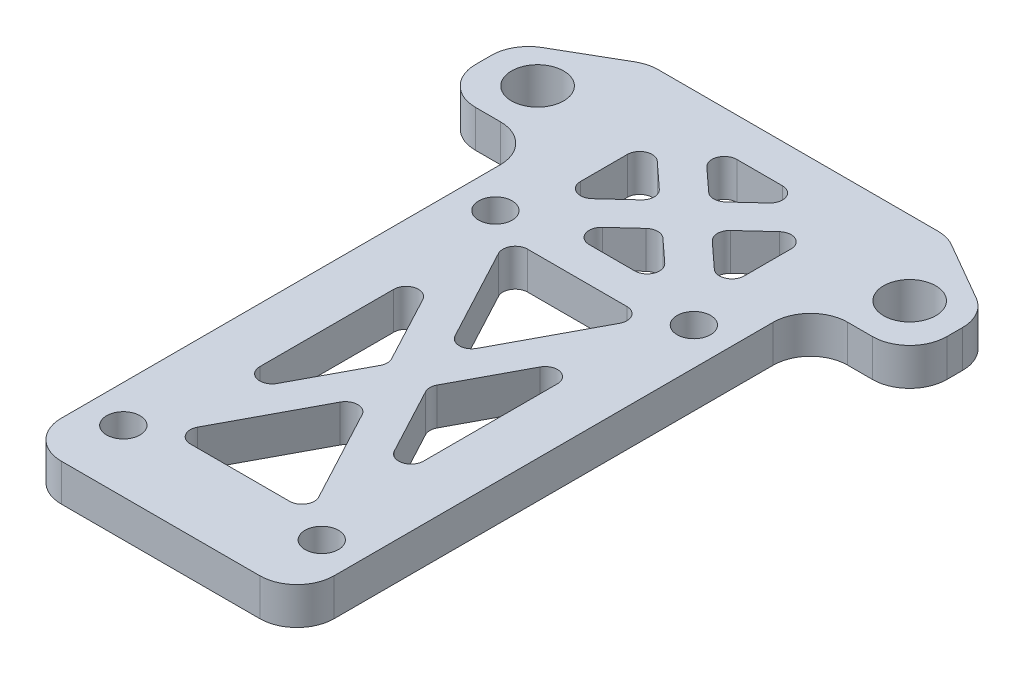
SolidWorks part; units mm, degrees
material "Thornel Mat VMA"
ref_plane "前视基准面" through (0, 0, 0) normal (0, 0, 1) x (1, 0, 0)
ref_plane "上视基准面" through (0, 0, 0) normal (0, 1, 0) x (1, 0, 0)
ref_plane "右视基准面" through (0, 0, 0) normal (1, 0, 0) x (0, 0, -1)
sketch "草图1" plane through (0, 0, 0) normal (0, 1, 0) x (1, 0, 0)
  line L0 (0, 6) -> (0, -45.4) construction
  line L2 (-12.0718, 6) -> (-19, 2)
  line L3 (-19, 2) -> (-19, -4)
  line L4 (-19, -4) -> (-11, -4)
  line L5 (-11, -4) -> (-11, -45.4)
  line L6 (-11, -45.4) -> (11, -45.4)
  line L7 (12.0718, 6) -> (19, 2)
  line L8 (19, 2) -> (19, -4)
  line L9 (19, -4) -> (11, -4)
  line L10 (11, -4) -> (11, -45.4)
  line L19 (12.0718, 6) -> (-12.0718, 6)
  circle A0 centre (-15, 0) radius 2.1
  circle A1 centre (15, 0) radius 2.1
  circle A2 centre (-8, -10.4) radius 1.35
  circle A3 centre (-8, -40.4) radius 1.35
  circle A4 centre (8, -10.4) radius 1.35
  circle A5 centre (8, -40.4) radius 1.35
  point P4 (-5, 53.1503)
  point P22 (0, 0)
  point P26 (11.54, 6.0449)
  point P27 (0, 6)
  dimension "D2" = 4.2
  dimension "D3" = 2.7
  dimension "D4" = 30
  dimension "D5" = 30
  dimension "D6" = 16
  dimension "D7" = 6.4
  dimension "D8" = 4
  dimension "D9" = 38
  dimension "D10" = 22
  dimension "D11" = 5
  dimension "D12" = 6
  dimension "D13" = 120
  dimension "D14" = 6
extrude "凸台-拉伸1" add sketch "草图1" along normal blind 3
sketch "草图2" plane through (0, 3, 0) normal (0, 1, 0) x (1, 0, 0)
  line L0 (-8, -10.4) -> (8, -40.4) construction
  line L1 (-6.7647, -9.7412) -> (9.2353, -39.7412)
  line L2 (-9.2353, -11.0588) -> (6.7647, -41.0588)
  line L3 (8, -10.4) -> (-8, -40.4) construction
  line L4 (9.2353, -11.0588) -> (-6.7647, -41.0588)
  line L5 (6.7647, -9.7412) -> (-9.2353, -39.7412)
  line L6 (-8, -10.4) -> (8, -10.4) construction
  line L7 (-8, -9) -> (8, -9)
  line L8 (-8, -11.8) -> (8, -11.8)
  line L9 (8, -10.4) -> (8, -40.4) construction
  line L10 (9.4, -10.4) -> (9.4, -40.4)
  line L11 (6.6, -10.4) -> (6.6, -40.4)
  line L12 (8, -40.4) -> (-8, -40.4) construction
  line L13 (8, -41.8) -> (-8, -41.8)
  line L14 (8, -39) -> (-8, -39)
  line L15 (-8, -40.4) -> (-8, -10.4) construction
  line L16 (-9.4, -40.4) -> (-9.4, -10.4)
  line L17 (-6.6, -40.4) -> (-6.6, -10.4)
  line L18 (-8, 4.3) -> (8, 4.3) construction
  line L19 (-8, 5.7) -> (8, 5.7)
  line L20 (-8, 2.9) -> (8, 2.9)
  line L21 (-8, 4.3) -> (-8, -10.4) construction
  line L22 (-6.6, 4.3) -> (-6.6, -10.4)
  line L23 (-9.4, 4.3) -> (-9.4, -10.4)
  line L24 (8, -10.4) -> (8, 4.3) construction
  line L25 (6.6, -10.4) -> (6.6, 4.3)
  line L26 (9.4, -10.4) -> (9.4, 4.3)
  line L27 (-8, 4.3) -> (8, -10.4) construction
  line L28 (-7.0528, 5.3309) -> (8.9472, -9.3691)
  line L29 (-8.9472, 3.2691) -> (7.0528, -11.4309)
  line L30 (8, 4.3) -> (-8, -10.4) construction
  line L31 (8.9472, 3.2691) -> (-7.0528, -11.4309)
  line L32 (7.0528, 5.3309) -> (-8.9472, -9.3691)
  line L34 (12.0718, 6) -> (-12.0718, 6) construction
  arc A0 (-6.7647, -9.7412) -> (-9.2353, -11.0588) centre (-8, -10.4) ccw
  arc A1 (6.7647, -41.0588) -> (9.2353, -39.7412) centre (8, -40.4) ccw
  arc A2 (9.2353, -11.0588) -> (6.7647, -9.7412) centre (8, -10.4) ccw
  arc A3 (-9.2353, -39.7412) -> (-6.7647, -41.0588) centre (-8, -40.4) ccw
  arc A4 (-8, -9) -> (-8, -11.8) centre (-8, -10.4) ccw
  arc A5 (8, -11.8) -> (8, -9) centre (8, -10.4) ccw
  arc A6 (9.4, -10.4) -> (6.6, -10.4) centre (8, -10.4) ccw
  arc A7 (6.6, -40.4) -> (9.4, -40.4) centre (8, -40.4) ccw
  arc A8 (8, -41.8) -> (8, -39) centre (8, -40.4) ccw
  arc A9 (-8, -39) -> (-8, -41.8) centre (-8, -40.4) ccw
  arc A10 (-9.4, -40.4) -> (-6.6, -40.4) centre (-8, -40.4) ccw
  arc A11 (-6.6, -10.4) -> (-9.4, -10.4) centre (-8, -10.4) ccw
  arc A12 (-8, 5.7) -> (-8, 2.9) centre (-8, 4.3) ccw
  arc A13 (8, 2.9) -> (8, 5.7) centre (8, 4.3) ccw
  arc A14 (-6.6, 4.3) -> (-9.4, 4.3) centre (-8, 4.3) ccw
  arc A15 (-9.4, -10.4) -> (-6.6, -10.4) centre (-8, -10.4) ccw
  arc A16 (6.6, -10.4) -> (9.4, -10.4) centre (8, -10.4) ccw
  arc A17 (9.4, 4.3) -> (6.6, 4.3) centre (8, 4.3) ccw
  arc A18 (-7.0528, 5.3309) -> (-8.9472, 3.2691) centre (-8, 4.3) ccw
  arc A19 (7.0528, -11.4309) -> (8.9472, -9.3691) centre (8, -10.4) ccw
  arc A20 (8.9472, 3.2691) -> (7.0528, 5.3309) centre (8, 4.3) ccw
  arc A21 (-8.9472, -9.3691) -> (-7.0528, -11.4309) centre (-8, -10.4) ccw
  point P4 (0, -25.4)
  point P9 (0, -25.4)
  point P20 (0, -10.4)
  point P25 (8, -25.4)
  point P32 (0, -40.4)
  point P39 (-8, -25.4)
  point P48 (0, 4.3)
  point P53 (-8, -3.05)
  point P60 (8, -3.05)
  point P67 (0, -3.05)
  point P74 (0, -3.05)
  dimension "D1" = 1.4
  dimension "D2" = 0.3
extrude "切除-拉伸1" cut sketch "草图2" against normal through all contours L32 L29 L22 | L32 L20 L28 | L25 L31 L28 | L29 L31 L7 | L8 L1 L5 | L17 L5 L2 | L14 L2 L4 | L11 L4 L1
fillet "R3 外缘圆角" radius 3 10 edges at (11, 1.5, 45.4) (11, 1.5, 4) (19, 1.5, 4) (19, 1.5, -2) (-19, 1.5, -2) (-19, 1.5, 4) (-11, 1.5, 4) (-11, 1.5, 45.4) (-12.0718, 1.5, -6) (12.0718, 1.5, -6)
fillet "R1 镂空圆角" radius 1 24 edges at (6.6, 1.5, 34.8) (6.6, 1.5, 16) (1.5867, 1.5, 25.4) (5.6667, 1.5, 39) (0, 1.5, 28.375) (-5.6667, 1.5, 39) (-6.6, 1.5, 34.8) (-1.5867, 1.5, 25.4) (-6.6, 1.5, 16) (0, 1.5, 22.425) (5.6667, 1.5, 11.8) (-5.6667, 1.5, 11.8) (4.4069, 1.5, -2.9) (0, 1.5, 1.1488) (-4.4069, 1.5, -2.9) (2.0693, 1.5, 3.05) (6.6, 1.5, -1.1126) (6.6, 1.5, 7.2126) (4.4069, 1.5, 9) (0, 1.5, 4.9512) (-4.4069, 1.5, 9) (-6.6, 1.5, 7.2126) (-2.0693, 1.5, 3.05) (-6.6, 1.5, -1.1126)
